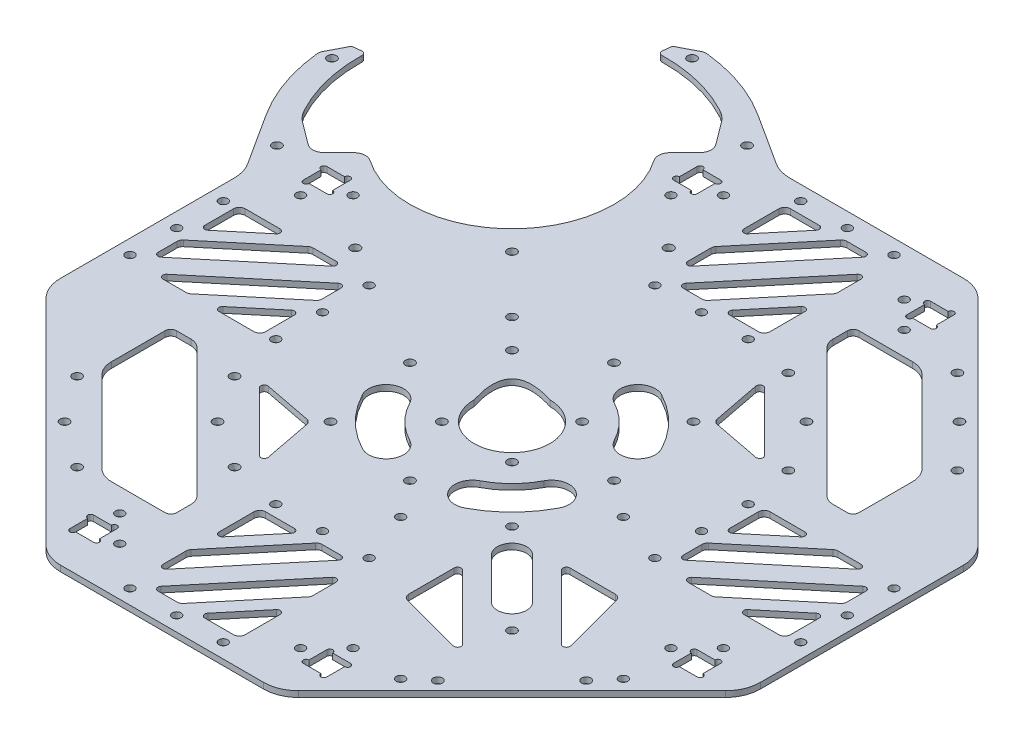
from build123d import *

# Parameters (mm, degrees)
SKETCH_1_R          = 1.5
SKETCH_1_R_2        = 1.55
SKETCH_1_R_3        = 1.6
EXTRUDE_1_DEPTH     = 2
SKETCH_2_R          = 1.55
CUT_EXTRUDE_1_DEPTH = 202.948659114
F_12MM_R            = 12
FILLET_1_2_R        = 1.2
FILLET_2_R          = 2
FILLET_4_R          = 4
FILLET_4_2_R        = 3
FILLET_5_R          = 5
FILLET_6_R          = 8


with BuildPart() as part:
    # 草图1 → 凸台-拉伸1 (new body)
    with BuildSketch(Plane(origin=(0, 0, 0), x_dir=(1, 0, 0), z_dir=(0, 1, 0))):
        with BuildLine():
            Line((-39.806132548, -120), (39.806132548, -120))
            Line((39.806132548, -120), (120, -39.806132548))
            Line((120, -39.806132548), (120, 39.806132548))
            Line((120, 39.806132548), (39.806132548, 120))
            Line((39.806132548, 120), (-28.287055437, 120))
            Line((-28.287055437, 120), (-49.044701087, 133.340469304))
            ThreePointArc((-49.044701087, 133.340469304), (-62.301720357, 139.748007741), (-76.70788631, 142.792263201))
            Line((-76.70788631, 142.792263201), (-84.067476167, 138.987758929))
            Line((-84.067476167, 138.987758929), (-84.462928082, 134.467722853))
            ThreePointArc((-84.462928082, 134.467722853), (-68.796441663, 132.830601516), (-54.320741271, 126.61988005))
            Line((-54.320741271, 126.61988005), (-45.315492706, 114.490639842))
            Line((-45.315492706, 114.490639842), (-55.245410262, 104.560722286))
            ThreePointArc((-55.245410262, 104.560722286), (-57.275649276, 57.275649276), (-104.560722286, 55.245410262))
            Line((-104.560722286, 55.245410262), (-114.490639842, 45.315492706))
            Line((-114.490639842, 45.315492706), (-126.61988005, 54.320741271))
            ThreePointArc((-126.61988005, 54.320741271), (-132.830601516, 68.796441663), (-134.467722853, 84.462928082))
            Line((-134.467722853, 84.462928082), (-138.987758929, 84.067476167))
            Line((-138.987758929, 84.067476167), (-142.792263201, 76.70788631))
            ThreePointArc((-142.792263201, 76.70788631), (-139.748007741, 62.301720357), (-133.340469304, 49.044701087))
            Line((-133.340469304, 49.044701087), (-120, 28.287055437))
            Line((-120, 28.287055437), (-120, -39.806132548))
            Line((-120, -39.806132548), (-39.806132548, -120))
        make_face()
        with BuildLine():
            Line((35.95, 99.45), (35.95, 105.55))
            ThreePointArc((35.95, 105.55), (34.95, 106.55), (35.95, 107.55))
            Line((35.95, 107.55), (42.05, 107.55))
            ThreePointArc((42.05, 107.55), (43.05, 108.55), (44.05, 107.55))
            Line((44.05, 107.55), (44.05, 101.45))
            ThreePointArc((44.05, 101.45), (45.05, 100.45), (44.05, 99.45))
            Line((44.05, 99.45), (37.95, 99.45))
            ThreePointArc((37.95, 99.45), (36.95, 98.45), (35.95, 99.45))
        make_face(mode=Mode.SUBTRACT)
        with BuildLine():
            Line((-37.95, 99.45), (-44.05, 99.45))
            ThreePointArc((-44.05, 99.45), (-45.05, 100.45), (-44.05, 101.45))
            Line((-44.05, 101.45), (-44.05, 107.55))
            ThreePointArc((-44.05, 107.55), (-43.05, 108.55), (-42.05, 107.55))
            Line((-42.05, 107.55), (-35.95, 107.55))
            ThreePointArc((-35.95, 107.55), (-34.95, 106.55), (-35.95, 105.55))
            Line((-35.95, 105.55), (-35.95, 99.45))
            ThreePointArc((-35.95, 99.45), (-36.95, 98.45), (-37.95, 99.45))
        make_face(mode=Mode.SUBTRACT)
        with BuildLine():
            Line((-99.45, 35.95), (-105.55, 35.95))
            ThreePointArc((-105.55, 35.95), (-106.55, 34.95), (-107.55, 35.95))
            Line((-107.55, 35.95), (-107.55, 42.05))
            ThreePointArc((-107.55, 42.05), (-108.55, 43.05), (-107.55, 44.05))
            Line((-107.55, 44.05), (-101.45, 44.05))
            ThreePointArc((-101.45, 44.05), (-100.45, 45.05), (-99.45, 44.05))
            Line((-99.45, 44.05), (-99.45, 37.95))
            ThreePointArc((-99.45, 37.95), (-98.45, 36.95), (-99.45, 35.95))
        make_face(mode=Mode.SUBTRACT)
        with BuildLine():
            Line((99.45, -35.95), (105.55, -35.95))
            ThreePointArc((105.55, -35.95), (106.55, -34.95), (107.55, -35.95))
            Line((107.55, -35.95), (107.55, -42.05))
            ThreePointArc((107.55, -42.05), (108.55, -43.05), (107.55, -44.05))
            Line((107.55, -44.05), (101.45, -44.05))
            ThreePointArc((101.45, -44.05), (100.45, -45.05), (99.45, -44.05))
            Line((99.45, -44.05), (99.45, -37.95))
            ThreePointArc((99.45, -37.95), (98.45, -36.95), (99.45, -35.95))
        make_face(mode=Mode.SUBTRACT)
        with BuildLine():
            ThreePointArc((-37.95, -99.45), (-36.95, -98.45), (-35.95, -99.45))
            Line((-35.95, -99.45), (-35.95, -105.55))
            ThreePointArc((-35.95, -105.55), (-34.95, -106.55), (-35.95, -107.55))
            Line((-35.95, -107.55), (-42.05, -107.55))
            ThreePointArc((-42.05, -107.55), (-43.05, -108.55), (-44.05, -107.55))
            Line((-44.05, -107.55), (-44.05, -101.45))
            ThreePointArc((-44.05, -101.45), (-45.05, -100.45), (-44.05, -99.45))
            Line((-44.05, -99.45), (-37.95, -99.45))
        make_face(mode=Mode.SUBTRACT)
        with BuildLine():
            ThreePointArc((35.95, -99.45), (36.95, -98.45), (37.95, -99.45))
            Line((37.95, -99.45), (44.05, -99.45))
            ThreePointArc((44.05, -99.45), (45.05, -100.45), (44.05, -101.45))
            Line((44.05, -101.45), (44.05, -107.55))
            ThreePointArc((44.05, -107.55), (43.05, -108.55), (42.05, -107.55))
            Line((42.05, -107.55), (35.95, -107.55))
            ThreePointArc((35.95, -107.55), (34.95, -106.55), (35.95, -105.55))
            Line((35.95, -105.55), (35.95, -99.45))
        make_face(mode=Mode.SUBTRACT)
        with Locations(Location((-16, -115, 0), (0, 0, 270))):
            Circle(SKETCH_1_R, mode=Mode.SUBTRACT)
        with Locations(Location((-31, -103.5, 0), (0, 0, 270))):
            Circle(SKETCH_1_R, mode=Mode.SUBTRACT)
        with Locations(Location((0, -115, 0), (0, 0, 270))):
            Circle(SKETCH_1_R, mode=Mode.SUBTRACT)
        with Locations(Location((16, -115, 0), (0, 0, 270))):
            Circle(SKETCH_1_R, mode=Mode.SUBTRACT)
        with Locations(Location((31, -103.5, 0), (0, 0, 270))):
            Circle(SKETCH_1_R, mode=Mode.SUBTRACT)
        with Locations(Location((90.863221382, 61.871843354, 0), (0, 0, 270))):
            Circle(SKETCH_1_R_2, mode=Mode.SUBTRACT)
        with Locations(Location((40, 94.5, 0), (0, 0, 270))):
            Circle(SKETCH_1_R, mode=Mode.SUBTRACT)
        with Locations(Location((61.871843354, 90.863221382, 0), (0, 0, 270))):
            Circle(SKETCH_1_R_2, mode=Mode.SUBTRACT)
        with Locations(Location((-88.071067812, -61.071067812, 0), (0, 0, 270))):
            Circle(SKETCH_1_R_2, mode=Mode.SUBTRACT)
        with Locations(Location((-61.071067812, -88.071067812, 0), (0, 0, 270))):
            Circle(SKETCH_1_R_2, mode=Mode.SUBTRACT)
        with Locations(Location((-40, -94.5, 0), (0, 0, 270))):
            Circle(SKETCH_1_R, mode=Mode.SUBTRACT)
        with Locations(Location((-34.071067812, -61.071067812, 0), (0, 0, 270))):
            Circle(SKETCH_1_R_2, mode=Mode.SUBTRACT)
        with Locations(Location((-16, -65, 0), (0, 0, 270))):
            Circle(SKETCH_1_R, mode=Mode.SUBTRACT)
        with Locations(Location((-61.071067812, -34.071067812, 0), (0, 0, 270))):
            Circle(SKETCH_1_R_2, mode=Mode.SUBTRACT)
        with BuildLine():
            ThreePointArc((-17.546447303, -33.706411661), (-26.870057685, -26.870057685), (-33.706411661, -17.546447303))
            ThreePointArc((-33.706411661, -17.546447303), (-31.154838341, -9.453890624), (-23.062281663, -12.005463944))
            ThreePointArc((-23.062281663, -12.005463944), (-18.384776311, -18.384776311), (-12.005463944, -23.062281663))
            ThreePointArc((-12.005463944, -23.062281663), (-9.453890624, -31.154838341), (-17.546447303, -33.706411661))
        make_face(mode=Mode.SUBTRACT)
        with Locations(Location((-65, -16, 0), (0, 0, 270))):
            Circle(SKETCH_1_R, mode=Mode.SUBTRACT)
        with Locations(Location((-65, 0, 0), (0, 0, 270))):
            Circle(SKETCH_1_R, mode=Mode.SUBTRACT)
        with Locations(Location((-12.02081528, -12.02081528, 0), (0, 0, 270))):
            Circle(SKETCH_1_R_2, mode=Mode.SUBTRACT)
        with Locations(Location((-35, 0, 0), (0, 0, 270))):
            Circle(SKETCH_1_R_2, mode=Mode.SUBTRACT)
        with Locations(Location((40, -94.5, 0), (0, 0, 270))):
            Circle(SKETCH_1_R, mode=Mode.SUBTRACT)
        with Locations(Location((0, -65, 0), (0, 0, 270))):
            Circle(SKETCH_1_R, mode=Mode.SUBTRACT)
        with Locations(Location((16, -65, 0), (0, 0, 270))):
            Circle(SKETCH_1_R, mode=Mode.SUBTRACT)
        with Locations(Location((57.275649276, -95.45941546, 0), (0, 0, 270))):
            Circle(SKETCH_1_R, mode=Mode.SUBTRACT)
        with Locations(Location((95.45941546, -57.275649276, 0), (0, 0, 270))):
            Circle(SKETCH_1_R, mode=Mode.SUBTRACT)
        with Locations(Location((9.192388155, -47.376154339, 0), (0, 0, 270))):
            Circle(SKETCH_1_R, mode=Mode.SUBTRACT)
        with Locations(Location((0, -35, 0), (0, 0, 270))):
            Circle(SKETCH_1_R_2, mode=Mode.SUBTRACT)
        with BuildLine():
            ThreePointArc((33.706411661, -17.546447303), (26.870057685, -26.870057685), (17.546447303, -33.706411661))
            ThreePointArc((17.546447303, -33.706411661), (9.453890624, -31.154838341), (12.005463944, -23.062281663))
            ThreePointArc((12.005463944, -23.062281663), (18.384776311, -18.384776311), (23.062281663, -12.005463944))
            ThreePointArc((23.062281663, -12.005463944), (31.154838341, -9.453890624), (33.706411661, -17.546447303))
        make_face(mode=Mode.SUBTRACT)
        with Locations(Location((12.02081528, -12.02081528, 0), (0, 0, 270))):
            Circle(SKETCH_1_R_2, mode=Mode.SUBTRACT)
        with BuildLine():
            ThreePointArc((0, 13), (9.192388155, -9.192388155), (-13, 0))
            add(Edge.make_bspline(
                [(-13, 0), (-18.955844123, 18.955844123), (0, 13)],
                knots=[0, 0, 0, 1, 1, 1], degree=2))
        make_face(mode=Mode.SUBTRACT)
        with Locations(Location((47.376154339, -9.192388155, 0), (0, 0, 270))):
            Circle(SKETCH_1_R, mode=Mode.SUBTRACT)
        with Locations(Location((35, 0, 0), (0, 0, 270))):
            Circle(SKETCH_1_R_2, mode=Mode.SUBTRACT)
        with Locations(Location((94.5, -40, 0), (0, 0, 270))):
            Circle(SKETCH_1_R, mode=Mode.SUBTRACT)
        with Locations(Location((65, -16, 0), (0, 0, 270))):
            Circle(SKETCH_1_R, mode=Mode.SUBTRACT)
        with Locations(Location((65, 0, 0), (0, 0, 270))):
            Circle(SKETCH_1_R, mode=Mode.SUBTRACT)
        with Locations(Location((-78.488852712, 24.748737342, 0), (0, 0, 270))):
            Circle(SKETCH_1_R_3, mode=Mode.SUBTRACT)
        with Locations(Location((-94.5, 40, 0), (0, 0, 270))):
            Circle(SKETCH_1_R, mode=Mode.SUBTRACT)
        with Locations(Location((-65, 16, 0), (0, 0, 270))):
            Circle(SKETCH_1_R, mode=Mode.SUBTRACT)
        with Locations(Location((-21.213203436, 21.213203436, 0), (0, 0, 270))):
            Circle(SKETCH_1_R_2, mode=Mode.SUBTRACT)
        with Locations(Location((-16, 65, 0), (0, 0, 270))):
            Circle(SKETCH_1_R, mode=Mode.SUBTRACT)
        with Locations(Location((-24.748737342, 78.488852712, 0), (0, 0, 270))):
            Circle(SKETCH_1_R_3, mode=Mode.SUBTRACT)
        with Locations(Location((-40, 94.5, 0), (0, 0, 270))):
            Circle(SKETCH_1_R, mode=Mode.SUBTRACT)
        with Locations(Location((12.02081528, 12.02081528, 0), (0, 0, 270))):
            Circle(SKETCH_1_R_2, mode=Mode.SUBTRACT)
        with Locations(Location((0, 35, 0), (0, 0, 270))):
            Circle(SKETCH_1_R_2, mode=Mode.SUBTRACT)
        with BuildLine():
            ThreePointArc((17.546447303, 33.706411661), (26.870057685, 26.870057685), (33.706411661, 17.546447303))
            ThreePointArc((33.706411661, 17.546447303), (31.154838341, 9.453890624), (23.062281663, 12.005463944))
            ThreePointArc((23.062281663, 12.005463944), (18.384776311, 18.384776311), (12.005463944, 23.062281663))
            ThreePointArc((12.005463944, 23.062281663), (9.453890624, 31.154838341), (17.546447303, 33.706411661))
        make_face(mode=Mode.SUBTRACT)
        with Locations(Location((0, 65, 0), (0, 0, 270))):
            Circle(SKETCH_1_R, mode=Mode.SUBTRACT)
        with Locations(Location((16, 65, 0), (0, 0, 270))):
            Circle(SKETCH_1_R, mode=Mode.SUBTRACT)
        with Locations(Location((32.880465325, 61.871843354, 0), (0, 0, 270))):
            Circle(SKETCH_1_R_2, mode=Mode.SUBTRACT)
        with Locations(Location((65, 16, 0), (0, 0, 270))):
            Circle(SKETCH_1_R, mode=Mode.SUBTRACT)
        with Locations(Location((61.871843354, 32.880465325, 0), (0, 0, 270))):
            Circle(SKETCH_1_R_2, mode=Mode.SUBTRACT)
        with Locations(Location((115, 16, 0), (0, 0, 270))):
            Circle(SKETCH_1_R, mode=Mode.SUBTRACT)
        with Locations(Location((115, 0, 0), (0, 0, 270))):
            Circle(SKETCH_1_R, mode=Mode.SUBTRACT)
        with Locations(Location((103.5, -31, 0), (0, 0, 270))):
            Circle(SKETCH_1_R, mode=Mode.SUBTRACT)
        with Locations(Location((115, -16, 0), (0, 0, 270))):
            Circle(SKETCH_1_R, mode=Mode.SUBTRACT)
        with Locations(Location((-103.5, 31, 0), (0, 0, 270))):
            Circle(SKETCH_1_R, mode=Mode.SUBTRACT)
        with Locations(Location((-115, 16, 0), (0, 0, 270))):
            Circle(SKETCH_1_R, mode=Mode.SUBTRACT)
        with Locations(Location((-115, -16, 0), (0, 0, 270))):
            Circle(SKETCH_1_R, mode=Mode.SUBTRACT)
        with Locations(Location((-115, 0, 0), (0, 0, 270))):
            Circle(SKETCH_1_R, mode=Mode.SUBTRACT)
        with Locations(Location((16, 115, 0), (0, 0, 270))):
            Circle(SKETCH_1_R, mode=Mode.SUBTRACT)
        with Locations(Location((0, 115, 0), (0, 0, 270))):
            Circle(SKETCH_1_R, mode=Mode.SUBTRACT)
        with Locations(Location((31, 103.5, 0), (0, 0, 270))):
            Circle(SKETCH_1_R, mode=Mode.SUBTRACT)
        with Locations(Location((-31, 103.5, 0), (0, 0, 270))):
            Circle(SKETCH_1_R, mode=Mode.SUBTRACT)
        with Locations(Location((-16, 115, 0), (0, 0, 270))):
            Circle(SKETCH_1_R, mode=Mode.SUBTRACT)
        with Locations(Location((-122.329473145, 41.71930009, 0), (0, 0, 270))):
            Circle(SKETCH_1_R_2, mode=Mode.SUBTRACT)
        with Locations(Location((-138.807484409, 77.056509281, 0), (0, 0, 270))):
            Circle(SKETCH_1_R_2, mode=Mode.SUBTRACT)
        with Locations(Location((-77.056509281, 138.807484409, 0), (0, 0, 270))):
            Circle(SKETCH_1_R_2, mode=Mode.SUBTRACT)
        with Locations(Location((-41.71930009, 122.329473145, 0), (0, 0, 270))):
            Circle(SKETCH_1_R_2, mode=Mode.SUBTRACT)
    extrude(amount=EXTRUDE_1_DEPTH)

    # 草图2 → 切除-拉伸1 (cut, through all)
    with BuildSketch(Plane(origin=(0, 2, 0), x_dir=(1, 0, 0), z_dir=(0, 1, 0))):
        Polygon((-17.5, -105.532825227), (12.944021022, -69), (2.944021022, -69), (-17.5, -93.532825227), align=None)
        Polygon((-17.5, -86.332825227), (-3.055978978, -69), (-17.5, -69), align=None)
        Polygon((17.5, -86.467174773), (17.5, -74.467174773), (-12.944021022, -111), (-2.944021022, -111), align=None)
        Polygon((17.5, -111), (17.5, -93.667174773), (3.055978978, -111), align=None)
        Polygon((-30.5, -86.5), (-30.5, -77.545916165), (-77.545916165, -30.5), (-86.5, -30.5), (-86.5, -54.156854249), (-54.156854249, -86.5), align=None)
        Polygon((30.5, 77.545916165), (77.545916165, 30.5), (86.5, 30.5), (86.5, 54.156854249), (54.156854249, 86.5), (30.5, 86.5), align=None)
        Polygon((-30.5, -56.156854249), (-34.648232278, -34.648232278), (-56.156854249, -30.5), align=None)
        Polygon((34.648232278, 34.648232278), (56.156854249, 30.5), (30.5, 56.156854249), align=None)
        Polygon((60.820508076, -77.791070824), (33.5, -50.470562748), (33.5, -70.470562748), align=None)
        Polygon((77.791070824, -60.820508076), (70.470562748, -33.5), (50.470562748, -33.5), align=None)
        Polygon((86.467174773, -17.5), (111, 2.944021022), (111, 12.944021022), (74.467174773, -17.5), align=None)
        Polygon((111, -17.5), (111, -3.055978978), (93.667174773, -17.5), align=None)
        Polygon((69, -12.944021022), (105.532825227, 17.5), (93.532825227, 17.5), (69, -2.944021022), align=None)
        Polygon((69, 3.055978978), (86.332825227, 17.5), (69, 17.5), align=None)
        Polygon((17.5, 105.532825227), (-12.944021022, 69), (-2.944021022, 69), (17.5, 93.532825227), align=None)
        Polygon((17.5, 86.332825227), (3.055978978, 69), (17.5, 69), align=None)
        Polygon((-17.5, 86.467174773), (-17.5, 74.467174773), (12.944021022, 111), (2.944021022, 111), align=None)
        Polygon((-17.5, 111), (-17.5, 93.667174773), (-3.055978978, 111), align=None)
        Polygon((-86.467174773, 17.5), (-111, -2.944021022), (-111, -12.944021022), (-74.467174773, 17.5), align=None)
        Polygon((-111, 17.5), (-111, 3.055978978), (-93.667174773, 17.5), align=None)
        Polygon((-69, 12.944021022), (-105.532825227, -17.5), (-93.532825227, -17.5), (-69, 2.944021022), align=None)
        Polygon((-69, -3.055978978), (-86.332825227, -17.5), (-69, -17.5), align=None)
        with BuildLine():
            Line((57.063517242, -49.99244943), (43.133513652, -36.062445841))
            ThreePointArc((43.133513652, -36.062445841), (36.062445841, -36.062445841), (36.062445841, -43.133513652))
            Line((36.062445841, -43.133513652), (49.99244943, -57.063517242))
            ThreePointArc((49.99244943, -57.063517242), (57.063517242, -57.063517242), (57.063517242, -49.99244943))
        make_face()
        with Locations(Location((-76.721085759, -76.721085759, 0), (0, 0, 270))):
            Circle(SKETCH_2_R)
        with Locations(Location((-50.487424177, -50.487424177, 0), (0, 0, 270))):
            Circle(SKETCH_2_R)
        with Locations(Location((62.014718626, -62.014718626, 0), (0, 0, 270))):
            Circle(SKETCH_2_R)
        with Locations(Location((64.136038969, -89.591883092, 0), (0, 0, 270))):
            Circle(SKETCH_2_R)
        with Locations(Location((89.591883092, -64.136038969, 0), (0, 0, 270))):
            Circle(SKETCH_2_R)
        with Locations(Location((-31.112698372, -31.112698372, 0), (0, 0, 90))):
            Circle(SKETCH_2_R)
        with Locations(Location((-50.487424177, 50.487424177, 0), (0, 0, 270))):
            Circle(SKETCH_2_R)
        with Locations(Location((-31.112698372, 31.112698372, 0), (0, 0, 90))):
            Circle(SKETCH_2_R)
        with Locations(Location((76.721085759, 76.721085759, 0), (0, 0, 270))):
            Circle(SKETCH_2_R)
        with Locations(Location((50.487424177, 50.487424177, 0), (0, 0, 270))):
            Circle(SKETCH_2_R)
        with Locations(Location((31.112698372, 31.112698372, 0), (0, 0, 90))):
            Circle(SKETCH_2_R)
        with Locations(Location((31.112698372, -31.112698372, 0), (0, 0, 270))):
            Circle(SKETCH_2_R)
    extrude(amount=-CUT_EXTRUDE_1_DEPTH, mode=Mode.SUBTRACT)

    # 12mm圆角
    f_12mm_edges = [part.edges().sort_by_distance(p)[0] for p in [
        (-126.61988005, 1, -54.320741271),
        (-54.320741271, 1, -126.61988005),
        (-28.287055437, 1, -120),
        (39.806132548, 1, -120),
        (120, 1, -39.806132548),
        (120, 1, 39.806132548),
        (39.806132548, 1, 120),
        (-39.806132548, 1, 120),
        (-120, 1, 39.806132548),
        (-120, 1, -28.287055437),
    ]]
    fillet(f_12mm_edges, radius=F_12MM_R)

    # 1.2圆角
    fillet_1_2_edges = [part.edges().sort_by_distance(p)[0] for p in [
        (-138.987758929, 1, -84.067476167),
        (-134.467722853, 1, -84.462928082),
        (-84.462928082, 1, -134.467722853),
        (-84.067476167, 1, -138.987758929),
        (-12.944021022, 1, 111),
        (17.5, 1, 74.467174773),
        (3.055978978, 1, 111),
        (17.5, 1, 93.667174773),
        (-17.5, 1, 86.332825227),
        (-3.055978978, 1, 69),
        (12.944021022, 1, 69),
        (-17.5, 1, 105.532825227),
        (111, 1, -12.944021022),
        (74.467174773, 1, 17.5),
        (111, 1, 3.055978978),
        (93.667174773, 1, 17.5),
        (86.332825227, 1, -17.5),
        (69, 1, -3.055978978),
        (69, 1, 12.944021022),
        (105.532825227, 1, -17.5),
        (12.944021022, 1, -111),
        (-17.5, 1, -74.467174773),
        (-3.055978978, 1, -111),
        (-17.5, 1, -93.667174773),
        (-12.944021022, 1, -69),
        (17.5, 1, -105.532825227),
        (17.5, 1, -86.332825227),
        (3.055978978, 1, -69),
        (60.820508076, 1, 77.791070824),
        (33.5, 1, 50.470562748),
        (77.791070824, 1, 60.820508076),
        (50.470562748, 1, 33.5),
        (30.5, 1, -56.156854249),
        (56.156854249, 1, -30.5),
        (-56.156854249, 1, 30.5),
        (-30.5, 1, 56.156854249),
        (-69, 1, -12.944021022),
        (-105.532825227, 1, 17.5),
        (-86.332825227, 1, 17.5),
        (-69, 1, 3.055978978),
        (-111, 1, -3.055978978),
        (-93.667174773, 1, -17.5),
        (-111, 1, 12.944021022),
        (-74.467174773, 1, -17.5),
    ]]
    fillet(fillet_1_2_edges, radius=FILLET_1_2_R)

    # 2圆角
    fillet_2_edges = [part.edges().sort_by_distance(p)[0] for p in [
        (-2.944021022, 1, 111),
        (17.5, 1, 86.467174773),
        (17.5, 1, 111),
        (-17.5, 1, 69),
        (2.944021022, 1, 69),
        (-17.5, 1, 93.532825227),
        (111, 1, -2.944021022),
        (86.467174773, 1, 17.5),
        (111, 1, 17.5),
        (69, 1, -17.5),
        (69, 1, 2.944021022),
        (93.532825227, 1, -17.5),
        (2.944021022, 1, -111),
        (-17.5, 1, -86.467174773),
        (-17.5, 1, -111),
        (-2.944021022, 1, -69),
        (17.5, 1, -93.532825227),
        (17.5, 1, -69),
        (-86.5, 1, 30.5),
        (-30.5, 1, 86.5),
        (30.5, 1, -86.5),
        (86.5, 1, -30.5),
        (33.5, 1, 70.470562748),
        (70.470562748, 1, 33.5),
        (34.648232278, 1, -34.648232278),
        (-34.648232278, 1, 34.648232278),
        (-69, 1, -2.944021022),
        (-93.532825227, 1, 17.5),
        (-69, 1, 17.5),
        (-111, 1, -17.5),
        (-111, 1, 2.944021022),
        (-86.467174773, 1, -17.5),
    ]]
    fillet(fillet_2_edges, radius=FILLET_2_R)

    # Fillet 4
    fillet_4_edges = [part.edges().sort_by_distance(p)[0] for p in [
        (-114.490639842, 1, -45.315492706),
        (-104.560722286, 1, -55.245410262),
        (-55.245410262, 1, -104.560722286),
        (-45.315492706, 1, -114.490639842),
    ]]
    fillet(fillet_4_edges, radius=FILLET_4_R)

    # Fillet 4 2
    fillet_4_2_edges = [part.edges().sort_by_distance(p)[0] for p in [
        (-142.792263201, 1, -76.70788631),
        (-76.70788631, 1, -142.792263201),
    ]]
    fillet(fillet_4_2_edges, radius=FILLET_4_2_R)

    # 圆角5
    fillet_5_edges = [part.edges().sort_by_distance(p)[0] for p in [
        (-77.545916165, 1, 30.5),
        (-30.5, 1, 77.545916165),
        (77.545916165, 1, -30.5),
        (30.5, 1, -77.545916165),
    ]]
    fillet(fillet_5_edges, radius=FILLET_5_R)

    # 圆角6
    fillet_6_edges = [part.edges().sort_by_distance(p)[0] for p in [
        (-54.156854249, 1, 86.5),
        (-86.5, 1, 54.156854249),
        (54.156854249, 1, -86.5),
        (86.5, 1, -54.156854249),
    ]]
    fillet(fillet_6_edges, radius=FILLET_6_R)


solid = part.part
